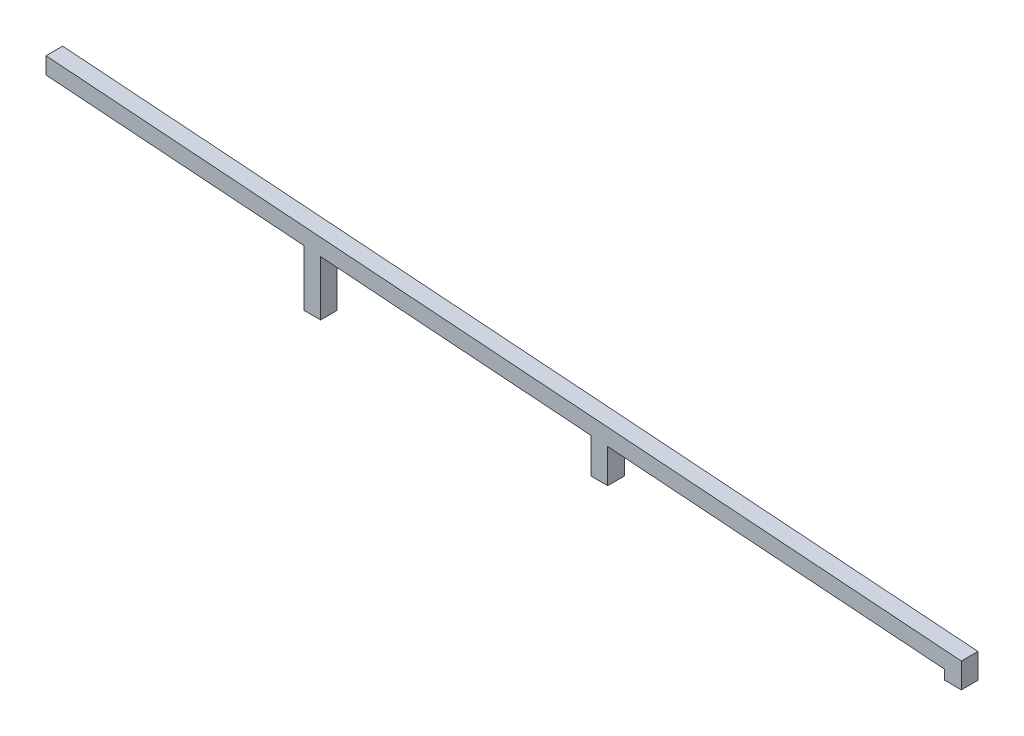
SolidWorks part; units mm, degrees
ref_plane "Front Plane" through (0, 0, 0) normal (0, 0, 1) x (1, 0, 0)
ref_plane "Top Plane" through (0, 0, 0) normal (0, 1, 0) x (1, 0, 0)
ref_plane "Right Plane" through (0, 0, 0) normal (1, 0, 0) x (0, 0, -1)
other "Configuration Table"
sketch "Sketch1" plane through (0, 0, 0) normal (0, 0, 1) x (1, 0, 0)
  line L0 (2200, 0) -> (2200, 60)
  line L1 (620, 0) -> (660, 0)
  line L2 (2200, 60) -> (0, 220)
  line L3 (0, 220) -> (0, 179.8944)
  line L8 (0, 179.8944) -> (620, 134.8034)
  line L9 (620, 134.8034) -> (620, 0)
  line L10 (660, 131.8944) -> (660, 0)
  line L11 (1350, 81.7125) -> (1350, 0)
  line L12 (1310, 84.6216) -> (1310, 0)
  line L13 (2160, 22.8034) -> (2160, 0)
  line L14 (1310, 0) -> (1350, 0)
  line L15 (2160, 0) -> (2200, 0)
  line L16 (1350, 81.7125) -> (2160, 22.8034)
  line L17 (660, 131.8944) -> (1310, 84.6216)
  point P17 (660, 65.9472)
  dimension "D2" = 2200
  dimension "D3" = 60
  dimension "D4" = 40
  dimension "D5" = 1350
  dimension "D6" = 40
  dimension "D7" = 40
  dimension "D8" = 40
  dimension "D9" = 650
extrude "Boss-Extrude1" add sketch "Sketch1" along normal blind 40
